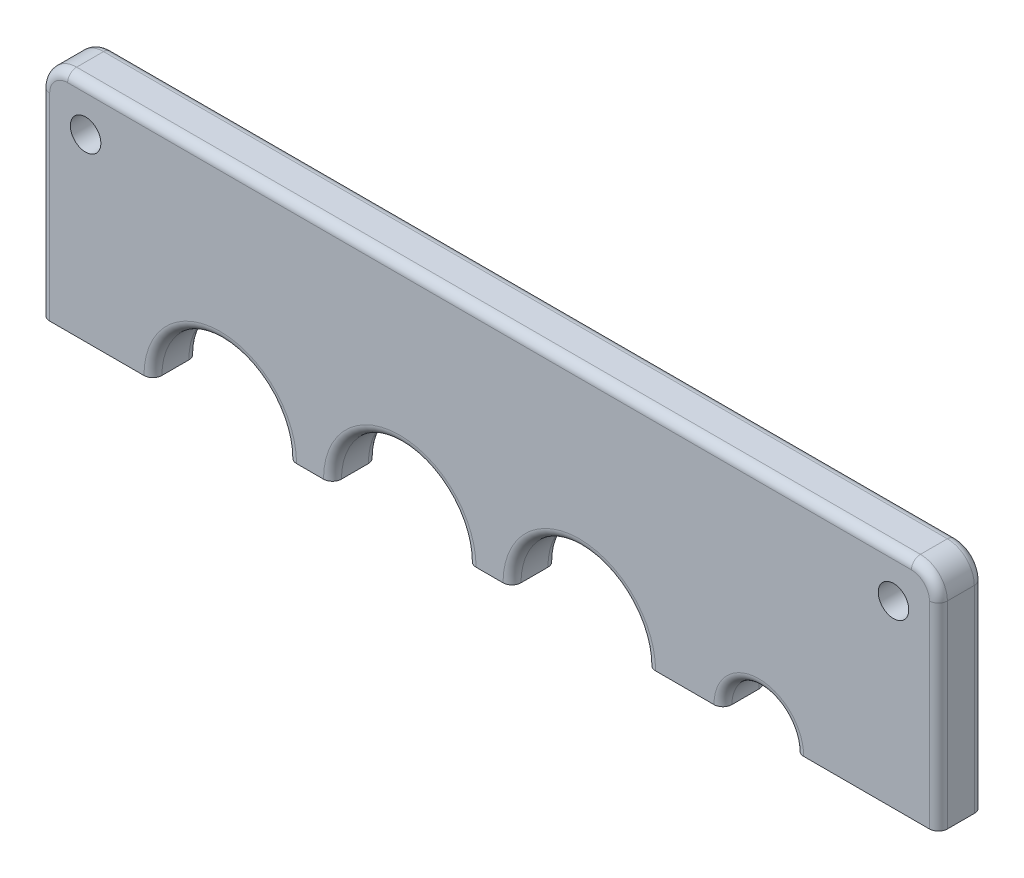
SolidWorks part; units mm, degrees
ref_plane "前视" through (0, 0, 0) normal (0, 0, 1) x (1, 0, 0)
ref_plane "上视" through (0, 0, 0) normal (0, 1, 0) x (1, 0, 0)
ref_plane "右视" through (0, 0, 0) normal (1, 0, 0) x (0, 0, -1)
sketch "草图1" plane through (0, 0, 0) normal (0, 0, 1) x (1, 0, 0)
  line L1 (0, 0) -> (100, 0)
  line L2 (0, 0) -> (0, 25)
  line L3 (0, 25) -> (100, 25)
  line L4 (100, 0) -> (100, 25)
  dimension "D1" = 25
  dimension "D2" = 100
extrude "凸台-拉伸1" add sketch "草图1" along normal blind 5
sketch "草图2" plane through (0, 0, 5) normal (0, 0, 1) x (1, 0, 0)
  line L0 (0, 0) -> (100, 0) construction
  line L1 (50, 25) -> (50, -16.1955) construction
  line L2 (100, 25) -> (0, 25) construction
  circle A0 centre (20, 0) radius 7.5
  circle A1 centre (40, 0) radius 7.5
  circle A2 centre (60, 0) radius 7.5
  circle A3 centre (80, 0) radius 4
  dimension "D1" = 8
  dimension "D3" = 15
  dimension "D4" = 15
  dimension "D2" = 20
  dimension "D5" = 60
extrude "切除-拉伸1" cut sketch "草图2" against normal through all
hole_wizard "M3 六角凹锥坑螺钉的锥形沉头孔1" positions "草图4" profile "草图3" countersink size "M3" standard "Iso" end condition through all
sketch "草图4" plane through (0, 0, 0) normal (0, 0, -1) x (-1, 0, 0)
  line L0 (-100, 25) -> (0, 25) construction
  line L1 (0, 25) -> (0, 0) construction
  line L2 (-100, 0) -> (-100, 25) construction
  point P0 (-5, 20)
  point P2 (-95, 20)
  dimension "D1" = 5
  dimension "D2" = 5
  dimension "D3" = 5
sketch "草图3" plane through (5, 20, 0) normal (1, 0, 0) x (0, 1, 0)
  line L0 (0, 0) -> (0, 5)
  line L1 (0, 5) -> (1.7, 5)
  line L2 (1.7, 5) -> (1.7, 1.66)
  line L3 (1.7, 1.66) -> (3.36, 0)
  line L5 (3.36, 0) -> (0, 0)
  line L6 (-1.7, 1.66) -> (-3.36, 0) construction
  line L11 (0, -6.35) -> (0, 107.95) construction
  dimension "通孔孔直径" = 3.4
  dimension "通孔孔深度" = 5
  dimension "近端锥形沉头孔直径" = 6.72
  dimension "近端锥形沉头孔角度" = 90
fillet "圆角1" radius 3 2 edges at (100, 25, 2.5) (0, 25, 2.5)
fillet "圆角2" radius 1 18 edges at (20, 7.5, 5) (40, 7.5, 5) (60, 7.5, 5) (80, 4, 5) (0, 11, 5) (0.8787, 24.1213, 5) (50, 25, 5) (99.1213, 24.1213, 5) (100, 11, 5) (0, 11, 0) (0.8787, 24.1213, 0) (50, 25, 0) (99.1213, 24.1213, 0) (100, 11, 0) (80, 4, 0) (60, 7.5, 0) (40, 7.5, 0) (20, 7.5, 0)
